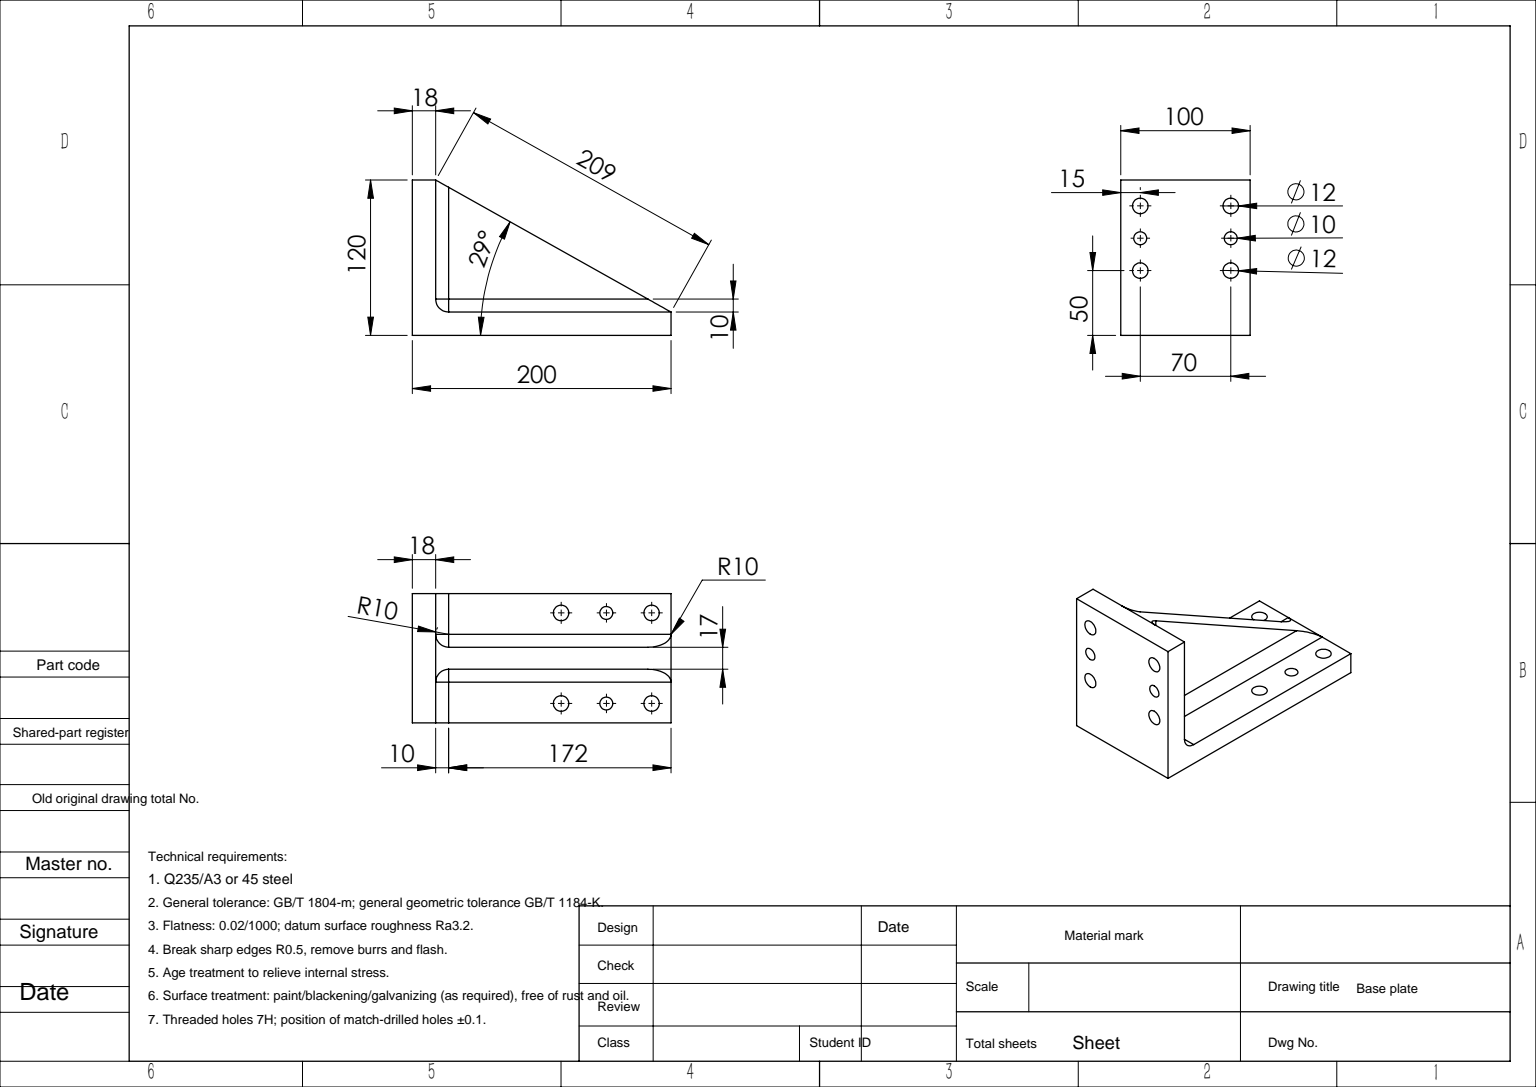
SolidWorks part; units mm, degrees
material "AISI 1045 钢，冷拔"
ref_plane "Front Plane" through (0, 0, 0) normal (0, 0, 1) x (1, 0, 0)
ref_plane "Top Plane" through (0, 0, 0) normal (0, 1, 0) x (1, 0, 0)
ref_plane "Right Plane" through (0, 0, 0) normal (1, 0, 0) x (0, 0, -1)
sketch "Sketch1" plane through (0, 0, 0) normal (1, 0, 0) x (0, 0, -1)
  line L0 (0, 0) -> (0, 200)
  line L1 (0, 200) -> (120, 200)
  line L2 (120, 200) -> (120, 182)
  line L3 (120, 182) -> (18, 182)
  line L4 (18, 182) -> (18, 0)
  line L5 (18, 0) -> (0, 0)
  dimension "D1" = 200
  dimension "D2" = 120
  dimension "D3" = 18
  dimension "D4" = 18
extrude "Boss-Extrude1" add sketch "Sketch1" along normal blind 100
fillet "Fillet1" radius 10 1 edges at (50, 182, -18)
ref_plane "Plane1" through (50, 0, 0) normal (1, 0, 0) x (0, 0, -1)
sketch "Sketch2" plane through (50, 0, 0) normal (1, 0, 0) x (0, 0, -1)
  line L0 (120, 182) -> (18, 0)
rib "Rib3" sketch "Sketch2" sketch "Sketch2" thickness 17 extrusion direction parallel to sketch draft on no parameters "D1"=17
fillet "Fillet2" radius 10 6 edges at (41.5, 86, -18) (41.5, 179.0711, -20.9289) (58.5, 86, -18) (58.5, 179.0711, -20.9289) (41.5, 182, -74) (58.5, 182, -74)
ref_plane "Plane2" through (0, 0, 0) normal (0, 0, 1) x (1, 0, 0)
sketch "Sketch3" plane through (0, 0, 0) normal (0, 0, 1) x (1, 0, 0)
  line L0 (0, 200) -> (0, 0) construction
  line L1 (50, 0) -> (100, 0) construction
  line L2 (100, 0) -> (100, 200) construction
  line L3 (100, 200) -> (50, 200) construction
  line L4 (50, 200) -> (50, 0) construction
  line L7 (15, 200) -> (0, 200) construction
  line L8 (100, 0) -> (0, 0) construction
  line L9 (25, 0) -> (0, 0) construction
  line L10 (0, 0) -> (0, 200) construction
  line L11 (0, 200) -> (15, 200) construction
  line L12 (15, 0) -> (15, 222.1111) construction
  circle A6 centre (15, 15) radius 6
  circle A7 centre (15, 50) radius 5
  circle A8 centre (15, 85) radius 6
  circle A9 centre (85, 15) radius 6
  circle A10 centre (85, 50) radius 5
  circle A11 centre (85, 85) radius 6
  dimension "D1" = 12
  dimension "D2" = 10
  dimension "D3" = 12
  dimension "D4" = 15
  dimension "D5" = 35
  dimension "D6" = 85
  dimension "D7" = 15
ref_plane "Plane3" through (0, 0, 0) normal (0, -1, 0) x (-1, 0, 0)
sketch "Sketch4" plane through (0, 0, 0) normal (0, -1, 0) x (1, 0, 0)
  line L0 (0, 0) -> (0, -18) construction
  line L1 (0, -18) -> (100, -18) construction
  line L2 (100, -18) -> (100, 0) construction
  line L3 (100, 0) -> (0, 0) construction
  line L4 (68.5, -18) -> (68.5, 0) construction
extrude "Cut-Extrude2" cut sketch "Sketch3" against normal through all
ref_plane "Plane4" through (0, 200, 0) normal (0, 1, 0) x (1, 0, 0)
sketch "Sketch7" plane through (0, 200, 0) normal (0, 1, 0) x (1, 0, 0)
  line L0 (15, 131.018) -> (15, -10.532) construction
  line L1 (0, 120) -> (0, 0) construction
  line L2 (100, 120) -> (0, 120) construction
  line L3 (50, -66) -> (50, 66) construction
  circle A0 centre (15, 100) radius 6
  circle A1 centre (15, 75) radius 5
  circle A2 centre (15, 50) radius 6
  circle A3 centre (85, 50) radius 6
  circle A4 centre (85, 75) radius 5
  circle A5 centre (85, 100) radius 6
  dimension "D2" = 20
  dimension "D3" = 25
  dimension "D4" = 70
  dimension "D1" = 15
extrude "Cut-Extrude3" cut sketch "Sketch7" against normal through all
